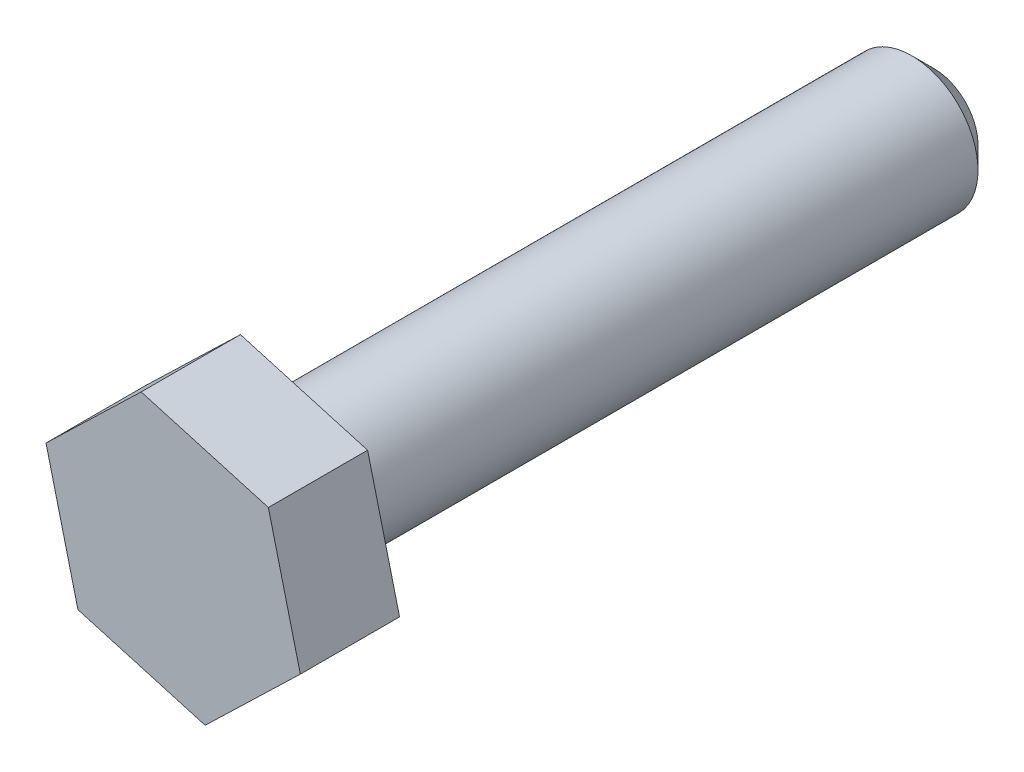
SolidWorks part; units mm, degrees
ref_plane "Front Plane" through (0, 0, 0) normal (0, 0, 1) x (1, 0, 0)
ref_plane "Top Plane" through (0, 0, 0) normal (0, 1, 0) x (1, 0, 0)
ref_plane "Right Plane" through (0, 0, 0) normal (1, 0, 0) x (0, 0, -1)
sketch "Sketch1" plane through (0, 0, 0) normal (0, 0, 1) x (1, 0, 0)
  circle A0 centre (0, 0) radius 6
  dimension "D1" = 12
extrude "Boss-Extrude1" add sketch "Sketch1" along normal blind 4.5
sketch "Sketch2" plane through (0, 0, 0) normal (0, 0, -1) x (-1, 0, 0)
  line L1 (4.3176, -4.1663) -> (5.7669, 1.656)
  line L2 (5.7669, 1.656) -> (1.4493, 5.8223)
  line L3 (1.4493, 5.8223) -> (-4.3176, 4.1663)
  line L4 (-4.3176, 4.1663) -> (-5.7669, -1.656)
  line L5 (-5.7669, -1.656) -> (-1.4493, -5.8223)
  line L6 (-1.4493, -5.8223) -> (4.3176, -4.1663)
  circle A0 centre (0, 0) radius 5.1962 construction
extrude "Cut-Extrude1" cut sketch "Sketch2" against normal blind 4.5 flip side to cut
sketch "Sketch3" plane through (0, 0, 0) normal (0, 0, -1) x (-1, 0, 0)
  circle A0 centre (0, 0) radius 3
  dimension "D1" = 6
extrude "Boss-Extrude2" add sketch "Sketch3" along normal blind 30
cosmetic thread "Cosmetic Thread1" parameters "D2"=5
chamfer "Chamfer1" distance 1 angle 45 1 edges at (-3, 0, -30)
